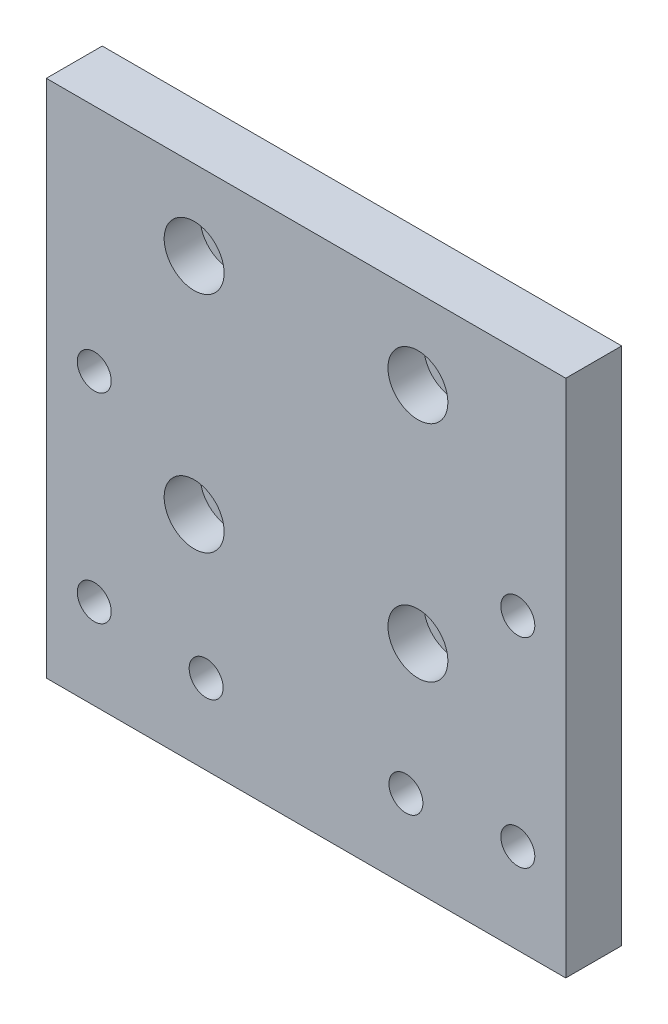
from build123d import *

# Parameters (mm, degrees)
SKETCH1_W                                          = 130
SKETCH1_H                                          = 130
BOSS_EXTRUDE1_DEPTH                                = 14
HOLE_SIZE_BASED_ON_SOCKET_HEAD_CAP_SCR_D           = 9
HOLE_SIZE_BASED_ON_SOCKET_HEAD_CAP_SCR_CBORE_D     = 15
HOLE_SIZE_BASED_ON_SOCKET_HEAD_CAP_SCR_CBORE_DEPTH = 9
M10_TAPPED_HOLE1_D                                 = 8.5
M10_TAPPED_HOLE2_D                                 = 8.5


with BuildPart() as part:
    # Sketch1 → Boss-Extrude1 (new body)
    with BuildSketch(Plane.XY):
        with Locations((65, 65)):
            Rectangle(SKETCH1_W, SKETCH1_H)
    extrude(amount=BOSS_EXTRUDE1_DEPTH)

    # Hole Size (%based on) Socket Head Cap Screw Type1 (through all)
    with Locations(Plane.XY.offset(14)):
        with Locations((37, 110), (93, 110), (93, 54), (37, 54)):
            CounterBoreHole(HOLE_SIZE_BASED_ON_SOCKET_HEAD_CAP_SCR_D / 2, HOLE_SIZE_BASED_ON_SOCKET_HEAD_CAP_SCR_CBORE_D / 2, HOLE_SIZE_BASED_ON_SOCKET_HEAD_CAP_SCR_CBORE_DEPTH)

    # M10 Tapped Hole1 (through all)
    with Locations(Plane(origin=(0, 0, 0), x_dir=(-1, 0, 0), z_dir=(0, 0, -1))):
        with Locations((-90, 20), (-40, 20)):
            Hole(M10_TAPPED_HOLE1_D / 2)

    # M10 Tapped Hole2 (through all)
    with Locations(Plane(origin=(0, 0, 0), x_dir=(-1, 0, 0), z_dir=(0, 0, -1))):
        with Locations((-118, 72.5), (-118, 22.5), (-12, 72.5), (-12, 22.5)):
            Hole(M10_TAPPED_HOLE2_D / 2)


solid = part.part
